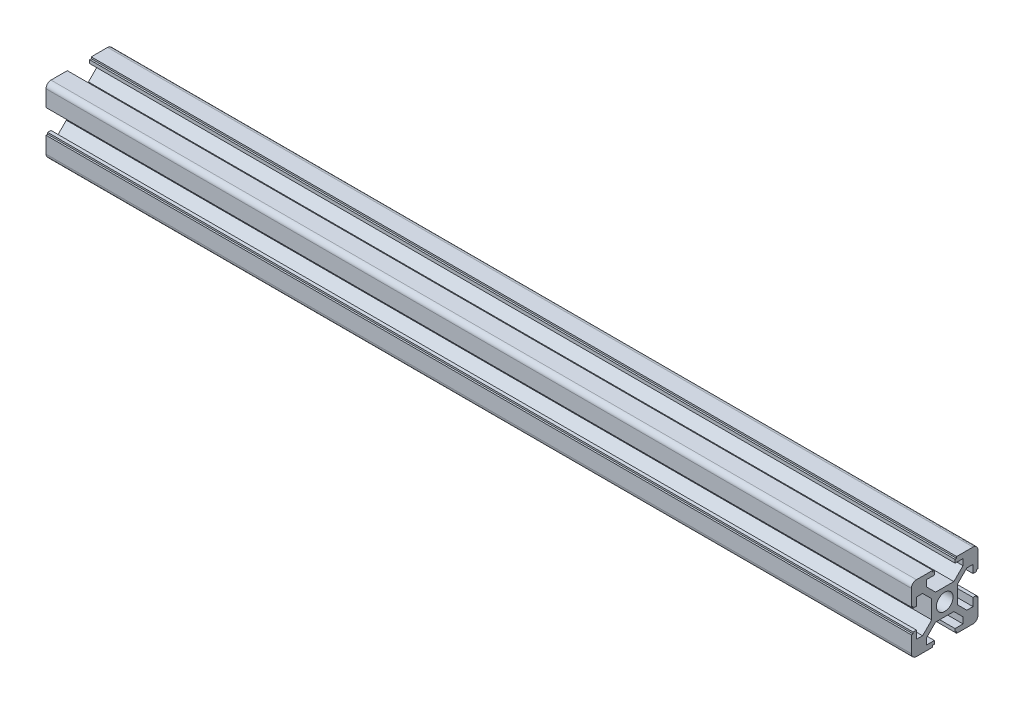
SolidWorks part; units mm, degrees
ref_plane "前视基准面" through (0, 0, 0) normal (0, 0, 1) x (1, 0, 0)
ref_plane "上视基准面" through (0, 0, 0) normal (0, 1, 0) x (1, 0, 0)
ref_plane "右视基准面" through (0, 0, 0) normal (1, 0, 0) x (0, 0, -1)
sketch "草图1" plane through (0, 0, 0) normal (0, 0, 1) x (1, 0, 0)
  line L0 (0, 0) -> (260, 0)
  dimension "D1" = 260
other "工业铝型材 20 X 20 X R1.5(1)"
ref_plane "基准面1" through (0, 0, 0) normal (1, 0, 0) x (0, 1, 0)
sketch "Sketch1" plane through (0, 0, 0) normal (1, 0, 0) x (0, 1, 0)
  line L0 (-3.6, 10) -> (-3.6, 9.5)
  line L1 (-3.6, 9.5) -> (-3.1, 9.5)
  line L2 (-3.1, 9.5) -> (-3.1, 8.5)
  line L3 (-3.1, 8.5) -> (-5.5, 8.5)
  line L4 (-8.5, -10) -> (-3.6, -10)
  line L5 (-10, -8.5) -> (-10, -3.6)
  line L6 (8.5, 10) -> (3.6, 10)
  line L7 (10, 8.5) -> (10, 3.6)
  line L8 (0, 14.8756) -> (0, 0) construction
  line L9 (0, 0) -> (14.1675, 0) construction
  line L10 (-5.5, 8.5) -> (-5.5, 6.65)
  line L11 (-5.5, 6.65) -> (-2.75, 3.9)
  line L12 (-2.75, 3.9) -> (2.75, 3.9)
  line L13 (5.5, 6.65) -> (2.75, 3.9)
  line L14 (5.5, 8.5) -> (5.5, 6.65)
  line L15 (3.1, 8.5) -> (5.5, 8.5)
  line L16 (3.1, 9.5) -> (3.1, 8.5)
  line L17 (3.6, 9.5) -> (3.1, 9.5)
  line L18 (3.6, 10) -> (3.6, 9.5)
  line L19 (-3.6, 10) -> (-8.5, 10)
  line L20 (10, 3.6) -> (9.5, 3.6)
  line L21 (9.5, 3.6) -> (9.5, 3.1)
  line L22 (9.5, 3.1) -> (8.5, 3.1)
  line L23 (8.5, 3.1) -> (8.5, 5.5)
  line L24 (8.5, 5.5) -> (6.65, 5.5)
  line L25 (6.65, 5.5) -> (3.9, 2.75)
  line L26 (3.9, 2.75) -> (3.9, -2.75)
  line L27 (6.65, -5.5) -> (3.9, -2.75)
  line L28 (8.5, -5.5) -> (6.65, -5.5)
  line L29 (8.5, -3.1) -> (8.5, -5.5)
  line L30 (9.5, -3.1) -> (8.5, -3.1)
  line L31 (9.5, -3.6) -> (9.5, -3.1)
  line L32 (10, -3.6) -> (9.5, -3.6)
  line L33 (3.6, -10) -> (3.6, -9.5)
  line L34 (3.6, -9.5) -> (3.1, -9.5)
  line L35 (3.1, -9.5) -> (3.1, -8.5)
  line L36 (3.1, -8.5) -> (5.5, -8.5)
  line L37 (5.5, -8.5) -> (5.5, -6.65)
  line L38 (5.5, -6.65) -> (2.75, -3.9)
  line L39 (2.75, -3.9) -> (-2.75, -3.9)
  line L40 (-5.5, -6.65) -> (-2.75, -3.9)
  line L41 (-5.5, -8.5) -> (-5.5, -6.65)
  line L42 (-3.1, -8.5) -> (-5.5, -8.5)
  line L43 (-3.1, -9.5) -> (-3.1, -8.5)
  line L44 (-3.6, -9.5) -> (-3.1, -9.5)
  line L45 (-3.6, -10) -> (-3.6, -9.5)
  line L46 (-10, -3.6) -> (-9.5, -3.6)
  line L47 (-9.5, -3.6) -> (-9.5, -3.1)
  line L48 (-9.5, -3.1) -> (-8.5, -3.1)
  line L49 (-8.5, -3.1) -> (-8.5, -5.5)
  line L50 (-8.5, -5.5) -> (-6.65, -5.5)
  line L51 (-6.65, -5.5) -> (-3.9, -2.75)
  line L52 (-3.9, -2.75) -> (-3.9, 2.75)
  line L53 (-6.65, 5.5) -> (-3.9, 2.75)
  line L54 (-8.5, 5.5) -> (-6.65, 5.5)
  line L55 (-8.5, 3.1) -> (-8.5, 5.5)
  line L56 (-9.5, 3.1) -> (-8.5, 3.1)
  line L57 (-9.5, 3.6) -> (-9.5, 3.1)
  line L58 (-10, 3.6) -> (-9.5, 3.6)
  line L59 (3.6, -10) -> (8.5, -10)
  line L60 (-10, 3.6) -> (-10, 8.5)
  line L61 (10, -3.6) -> (10, -8.5)
  circle A0 centre (0, 0) radius 2.5
  arc A1 (-10, 8.5) -> (-8.5, 10) centre (-8.5, 8.5) cw
  arc A2 (10, 8.5) -> (8.5, 10) centre (8.5, 8.5) ccw
  arc A3 (-8.5, -10) -> (-10, -8.5) centre (-8.5, -8.5) cw
  arc A4 (8.5, -10) -> (10, -8.5) centre (8.5, -8.5) ccw
  point P0 (-10, 0)
  point P1 (10, 0)
  point P2 (0, 10)
  point P3 (0, -10)
  point P4 (0, 0)
  point P5 (-10, -10)
  point P6 (10, -10)
  point P7 (10, 10)
  point P8 (-10, 10)
  point P13 (0, 0)
  point P36 (-10, 10)
  point P39 (10, 10)
  dimension "D1" = 11
  dimension "D2" = 20
  dimension "D3" = 6.2
  dimension "D4" = 7.2
  dimension "D5" = 6.1
  dimension "D6" = 5
  dimension "D7" = 1.5
  dimension "D8" = 45
  dimension "D9" = 0.5
  dimension "D10" = 1
  dimension "D11" = 5.5
